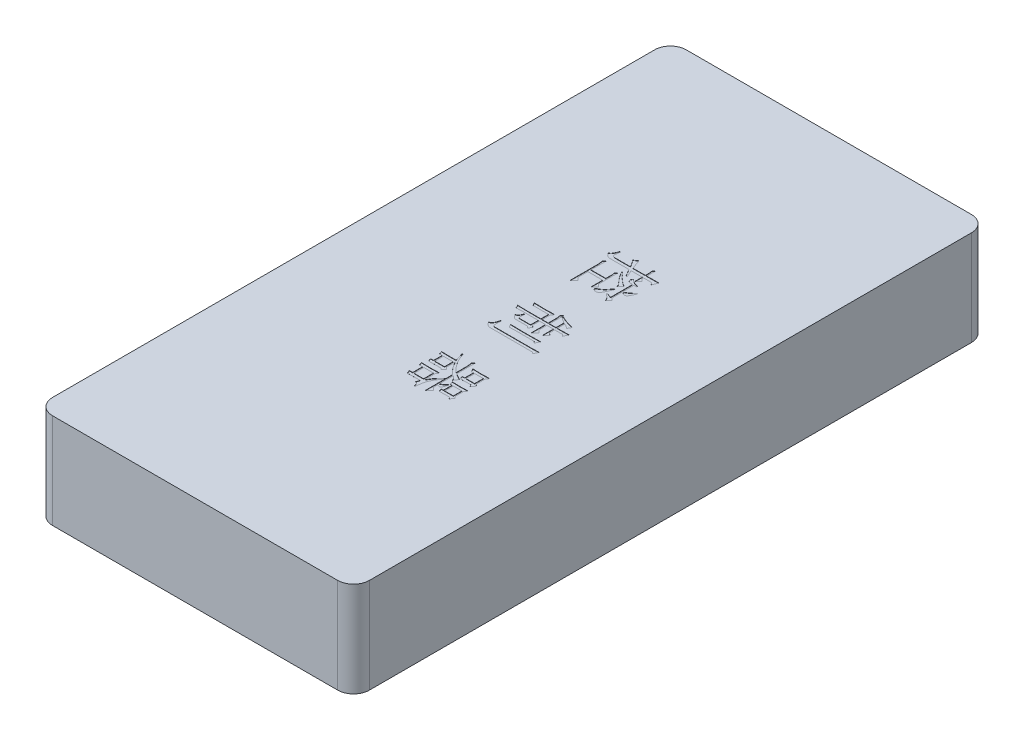
SolidWorks part; units mm, degrees
ref_plane "前视" through (0, 0, 0) normal (0, 0, 1) x (1, 0, 0)
ref_plane "上视" through (0, 0, 0) normal (0, 1, 0) x (1, 0, 0)
ref_plane "右视" through (0, 0, 0) normal (1, 0, 0) x (0, 0, -1)
sketch "草图1" plane through (0, 0, 0) normal (0, 1, 0) x (1, 0, 0)
  line L1 (-50, 100) -> (50, 100)
  line L2 (-50, 100) -> (-50, -100)
  line L3 (-50, -100) -> (50, -100)
  line L4 (50, 100) -> (50, -100)
  line L5 (-50, 100) -> (50, -100) construction
  line L6 (-50, -100) -> (50, 100) construction
  point P0 (0, 0)
  dimension "D1" = 100
  dimension "D2" = 200
extrude "凸台-拉伸1" add sketch "草图1" along normal blind 30
sketch "草图2" plane through (0, 30, 0) normal (0, 1, 0) x (1, 0, 0)
  line L0 (0, 500) -> (0, -500) construction
  line L1 (-500, 0) -> (500, 0) construction
  text T0 "控 制 器" font "新宋体" height 12
extrude "切除-拉伸1" cut sketch "草图2" against normal blind 0.1
fillet "圆角1" radius 5 4 edges at (-50, 15, -100) (-50, 15, 100) (50, 15, 100) (50, 15, -100)
